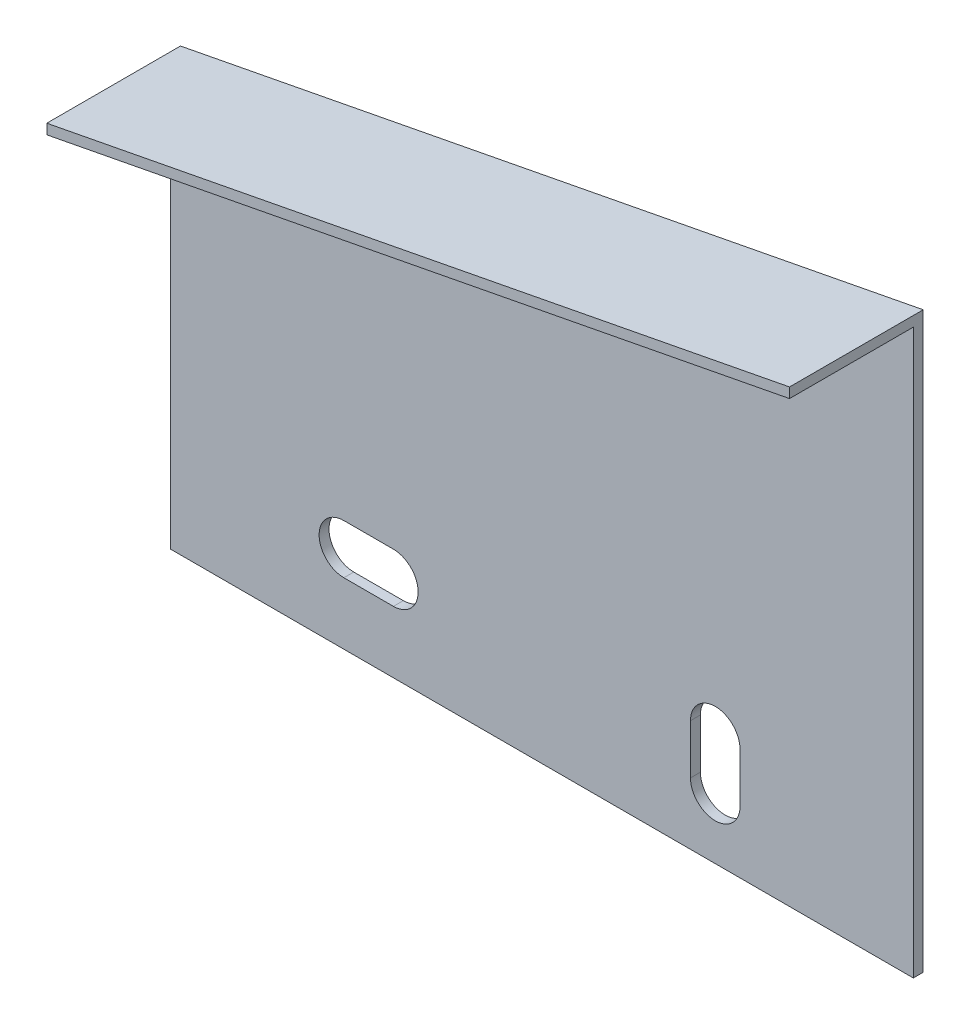
SolidWorks part; units mm, degrees
ref_plane "Front Plane" through (0, 0, 0) normal (0, 0, 1) x (1, 0, 0)
ref_plane "Top Plane" through (0, 0, 0) normal (0, 1, 0) x (1, 0, 0)
ref_plane "Right Plane" through (0, 0, 0) normal (1, 0, 0) x (0, 0, -1)
other "Configuration Table"
sketch "Sketch1" plane through (0, 0, 0) normal (0, 0, 1) x (1, 0, 0)
  line L0 (0, 174) -> (300, 231.7425)
  line L1 (300, 231.7425) -> (300, 0)
  line L2 (300, 0) -> (0, 0)
  line L3 (0, 0) -> (0, 174)
  line L4 (70, 45) -> (90, 45)
  line L5 (90, 25) -> (70, 25)
  line L6 (230, 45) -> (230, 25)
  line L7 (210, 25) -> (210, 45)
  arc A0 (90, 25) -> (90, 45) centre (90, 35) ccw
  arc A1 (70, 45) -> (70, 25) centre (70, 35) ccw
  arc A2 (210, 25) -> (230, 25) centre (220, 25) ccw
  arc A3 (230, 45) -> (210, 45) centre (220, 45) ccw
  dimension "D1" = 10
  dimension "D2" = 70
  dimension "D3" = 220
  dimension "D4" = 300
  dimension "D5" = 35
  dimension "D6" = 174
  dimension "D7" = 231.7425
extrude "Boss-Extrude1" add sketch "Sketch1" along normal blind 4
sketch "Sketch2" plane through (0, 0, 4) normal (0, 0, 1) x (1, 0, 0)
  line L1 (0, 174) -> (0, 0) construction
  line L2 (21.1634, 174) -> (300, 227.6691)
  line L3 (300, 0) -> (300, 231.7425) construction
  line L4 (300, 227.6691) -> (300, 231.7425)
  line L5 (300, 231.7425) -> (0, 174)
  line L7 (21.1634, 174) -> (300, 174) construction
  line L8 (0, 174) -> (0, 169.9266)
  line L9 (0, 169.9266) -> (300, 169.9266) construction
  line L10 (300, 174) -> (300, 169.9266) construction
  line L11 (0, 174) -> (21.1634, 174) construction
  line L12 (0, 169.9266) -> (21.1634, 174)
  dimension "D1" = 4
extrude "Boss-Extrude2" add sketch "Sketch2" along normal blind 50
